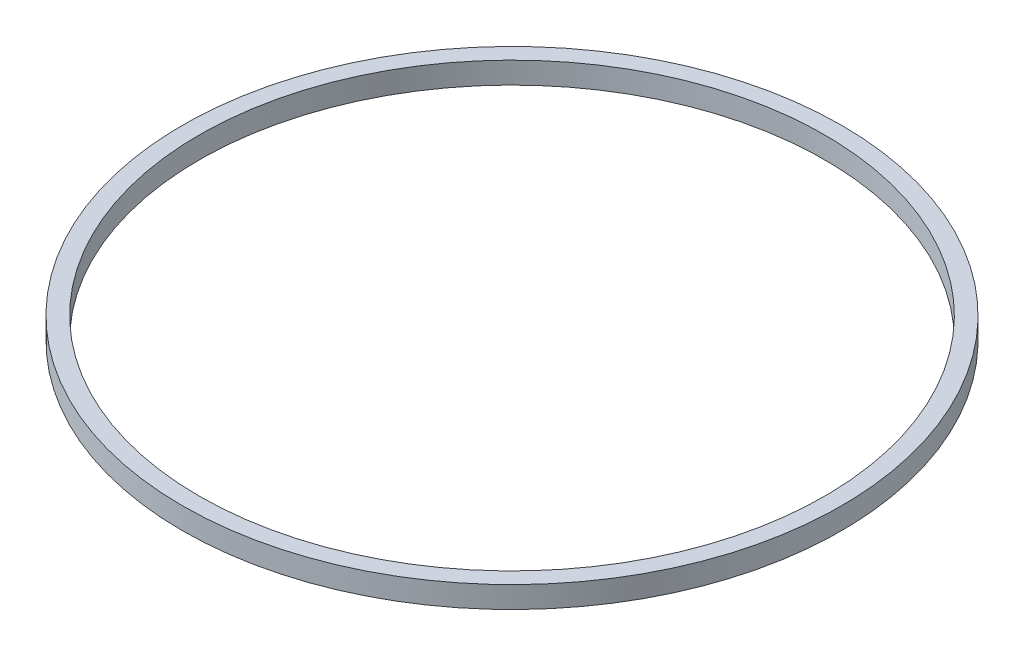
from build123d import *

# Parameters (mm, degrees)
SKETCH_1_R      = 305
SKETCH_1_R_2    = 289.5
EXTRUDE_1_DEPTH = 20


with BuildPart() as part:
    # 草图1 → 凸台-拉伸1 (new body)
    with BuildSketch(Plane(origin=(0, 0, 0), x_dir=(1, 0, 0), z_dir=(0, 1, 0))):
        with Locations(Location((0, 0, 0), (0, 0, 270))):
            Circle(SKETCH_1_R)
        with Locations(Location((0, 0, 0), (0, 0, 270))):
            Circle(SKETCH_1_R_2, mode=Mode.SUBTRACT)
    extrude(amount=EXTRUDE_1_DEPTH)


solid = part.part
